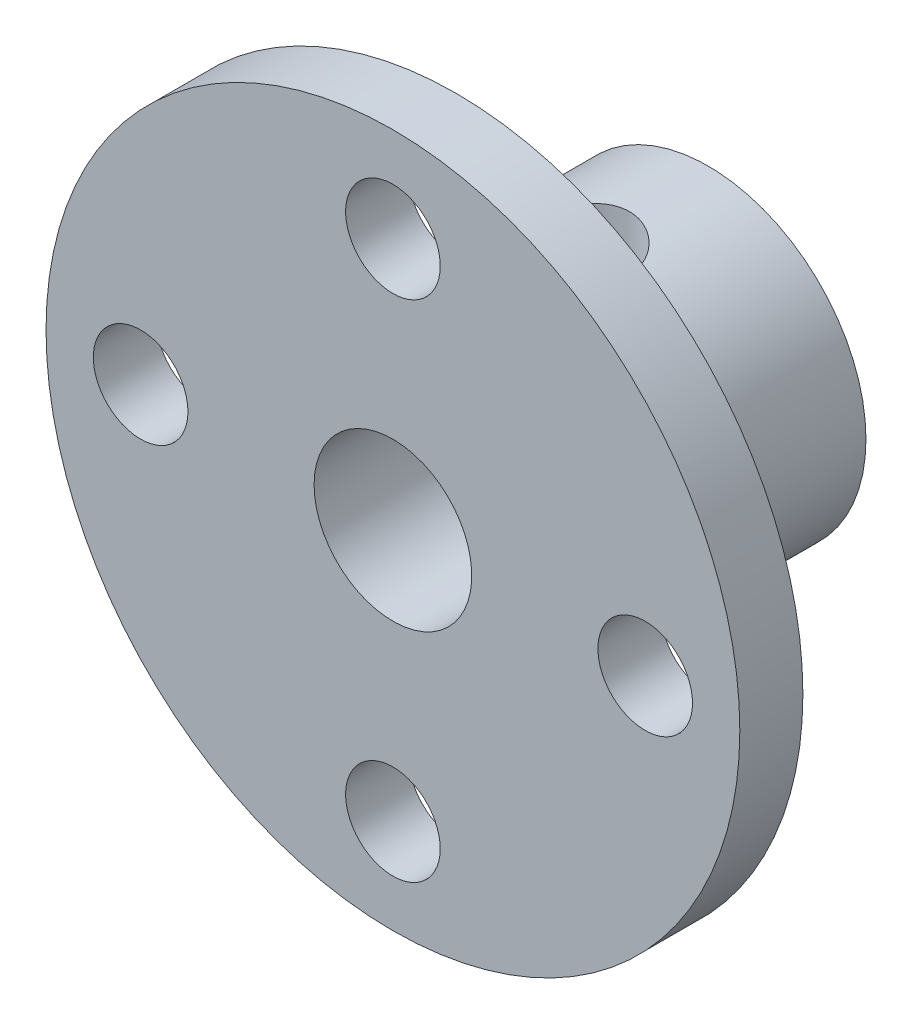
SolidWorks part; units mm, degrees
material "1060 合金"
ref_plane "Front Plane" through (0, 0, 0) normal (0, 0, 1) x (1, 0, 0)
ref_plane "Top Plane" through (0, 0, 0) normal (0, 1, 0) x (1, 0, 0)
ref_plane "Right Plane" through (0, 0, 0) normal (1, 0, 0) x (0, 0, -1)
other "Configuration Table"
sketch "Sketch1" plane through (0, 0, 0) normal (0, 0, 1) x (1, 0, 0)
  circle A0 centre (0, 0) radius 11
  dimension "D1" = 22
extrude "Boss-Extrude1" add sketch "Sketch1" along normal blind 2
sketch "Sketch2" plane through (0, 0, 0) normal (0, 0, -1) x (-1, 0, 0)
  circle A0 centre (0, 0) radius 5
  dimension "D1" = 10
extrude "Boss-Extrude2" add sketch "Sketch2" along normal blind 8
sketch "Sketch3" plane through (0, 0, -8) normal (0, 0, -1) x (-1, 0, 0)
  circle A0 centre (0, 0) radius 2.5
  dimension "D1" = 5
extrude "Cut-Extrude1" cut sketch "Sketch3" against normal through all
sketch "Sketch4" plane through (0, 0, 2) normal (0, 0, 1) x (1, 0, 0)
  circle A0 centre (0, 0) radius 8 construction
  circle A1 centre (0, -8) radius 1.5
  circle A4 centre (-8, 0) radius 1.5
  circle A5 centre (0, 8) radius 1.5
  circle A6 centre (8, 0) radius 1.5
  point P11 (-1.299, 2.25)
  point P15 (0, 0)
  dimension "D1" = 16
  dimension "D2" = 3
  dimension "D3" = 4
extrude "Cut-Extrude2" cut sketch "Sketch4" against normal through all
sketch "Sketch5" plane through (0, 0, 0) normal (0, 1, 0) x (1, 0, 0)
  line L0 (0, 0) -> (0, 8) construction
  line L1 (11, 0) -> (-11, 0) construction
  line L2 (5, 8) -> (-5, 8) construction
  circle A0 centre (0, 4) radius 1.5
  dimension "D1" = 3
extrude "Cut-Extrude3" cut sketch "Sketch5" against normal mid plane 14
